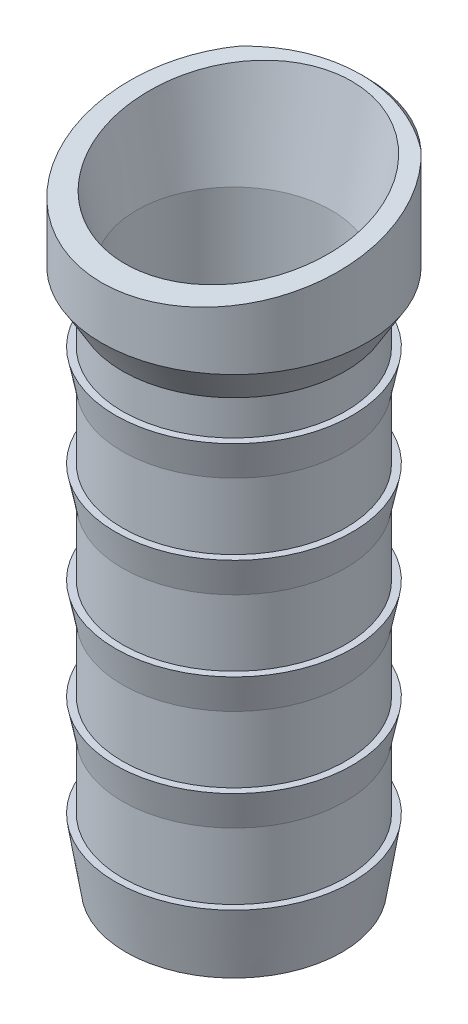
SolidWorks part; units mm, degrees
material "普通碳钢"
ref_plane "前视基准面" through (0, 0, 0) normal (0, 0, 1) x (1, 0, 0)
ref_plane "上视基准面" through (0, 0, 0) normal (0, 1, 0) x (1, 0, 0)
ref_plane "右视基准面" through (0, 0, 0) normal (1, 0, 0) x (0, 0, -1)
sketch "草图1" plane through (0, 0, 0) normal (0, 0, 1) x (1, 0, 0)
  line L0 (0, 92.5) -> (0, -92.5)
  line L1 (0, -92.5) -> (31, -92.5)
  line L2 (31, -92.5) -> (34, -73.5)
  line L3 (34, -73.5) -> (32, -73.5)
  line L5 (34, -44.5) -> (32, -44.5)
  line L11 (0, 92.5) -> (36, 92.5)
  line L23 (32, 42.5) -> (32, 52.5)
  line L24 (38, 90.5) -> (38, 62.5)
  line L25 (32, 52.5) -> (38, 62.5)
  line L26 (36, 92.5) -> (38, 90.5)
  line L30 (32, -73.5) -> (32, -54.5)
  line L31 (32, -54.5) -> (34, -44.5)
  line L32 (32, -25.5) -> (34, -15.5)
  line L33 (34, -15.5) -> (32, -15.5)
  line L34 (32, -44.5) -> (32, -25.5)
  line L35 (34, 13.5) -> (32, 13.5)
  line L36 (32, -15.5) -> (32, 3.5)
  line L37 (32, 3.5) -> (34, 13.5)
  line L38 (32, 32.5) -> (34, 42.5)
  line L39 (34, 42.5) -> (32, 42.5)
  line L40 (32, 13.5) -> (32, 32.5)
  point P4 (0, 0)
  point P16 (38, 92.5)
  dimension "D1" = 185
  dimension "D2" = 31
  dimension "D3" = 34
  dimension "D4" = 2
  dimension "D5" = 19
  dimension "D6" = 19
  dimension "D7" = 2
  dimension "D8" = 10
  dimension "D9" = 2
  dimension "D10" = 10
  dimension "D11" = 19
  dimension "D12" = 2
  dimension "D13" = 10
  dimension "D14" = 19
  dimension "D15" = 10
  dimension "D16" = 10
  dimension "D17" = 19
  dimension "D20" = 34
  dimension "D22" = 10
  dimension "D23" = 38
revolve "旋转1" add sketch "草图1" angle 360 about L0
sketch "草图2" plane through (0, 92.5, 0) normal (0, 1, 0) x (1, 0, 0)
  circle A0 centre (0, 0) radius 28
  dimension "D1" = 56
extrude "切除-拉伸1" cut sketch "草图2" against normal up to surface (185 mm away) up to face at (0, -92.5, 31)
ref_plane "基准面1" through (0, 62.5, 0) normal (0, 1, 0) x (-1, 0, 0)
sketch "草图3" plane through (0, 62.5, 0) normal (0, 1, 0) x (-1, 0, 0)
  circle A0 centre (0, 0) radius 28
  dimension "D1" = 56
sketch "草图4" plane through (0, 92.5, 0) normal (0, 1, 0) x (1, 0, 0)
  circle A0 centre (0, 0) radius 34
  dimension "D1" = 68
loft "切除-放样1" cut profiles "草图4", "草图3"
sketch "草图5" plane through (0, 0, 0) normal (1, 0, 0) x (0, 0, -1)
  line L0 (-38, 77.5) -> (38, 92.5)
  line L1 (-38, 90.5) -> (-38, 62.5) construction
  line L2 (38, 62.5) -> (38, 90.5) construction
  line L3 (34, 92.5) -> (-34, 92.5) construction
  line L4 (38, 92.5) -> (-38, 92.5)
  line L5 (-38, 92.5) -> (-38, 77.5)
  dimension "D1" = 15
extrude "切除-拉伸2" cut sketch "草图5" against normal mid plane 100
sketch "草图6" plane through (0, 81.813, 16.1473) normal (0, 0.9811, 0.1936) x (1, 0, 0)
  point P2 (0, 17.7685)
